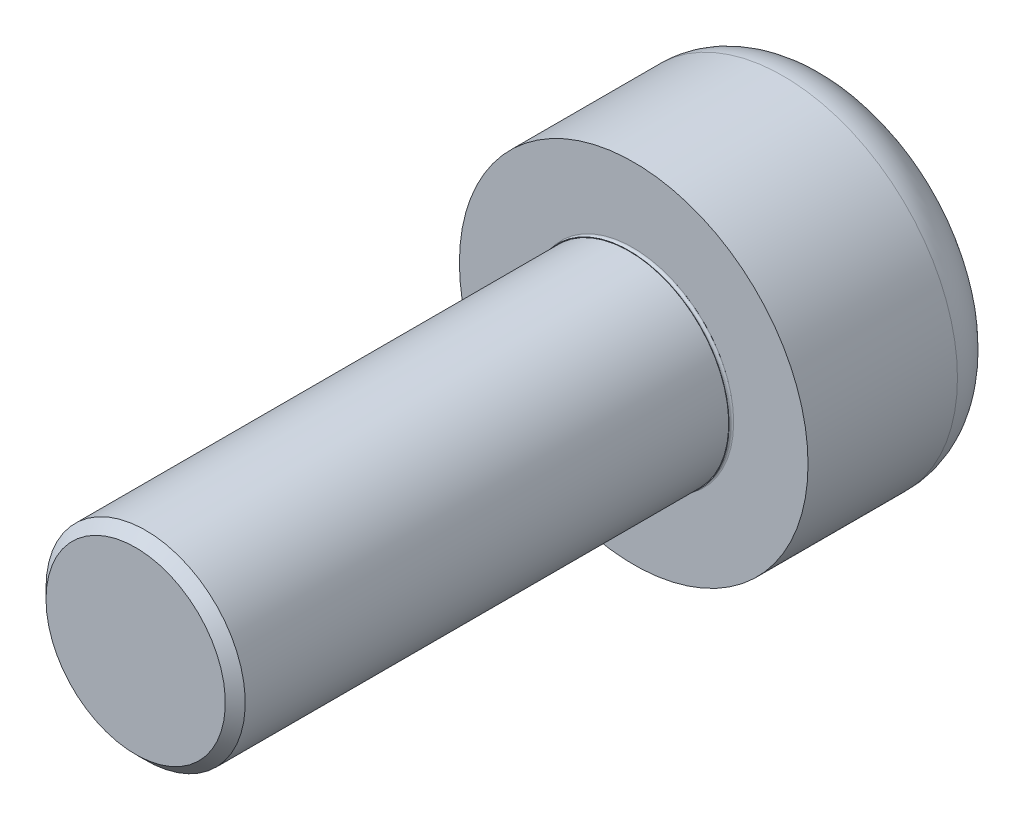
from build123d import *

# Parameters (mm, degrees)
CUT_EXTRUDE1_DEPTH = 0.75


with BuildPart() as part:
    # Logo3_bib1 → Revolve1 (revolve)
    with BuildSketch(Plane(origin=(0, 0, 0), x_dir=(-1, 0, 0), z_dir=(0, -1, 0))):
        with BuildLine():
            Line((0, -5), (0, 2))
            Line((0, 2), (1.25, 2))
            ThreePointArc((1.25, 2), (1.603553391, 1.853553391), (1.75, 1.5))
            Line((1.75, 1.5), (1.75, 0))
            Line((1.75, 0), (1, 0))
            Line((1, 0), (1, -0.01))
            Line((1, -0.01), (1.013425636, -0.01))
            ThreePointArc((1.013425636, -0.01), (0.993729481, -0.026527036), (1.006585234, -0.048793852))
            Line((1.006585234, -0.048793852), (1, -0.046397023))
            Line((1, -0.046397023), (1, -4.9))
            Line((1, -4.9), (0.9, -5))
            Line((0.9, -5), (0, -5))
        make_face()
    revolve(axis=Axis((0, 0, -10.585154653), (0, 0, 1)))

    # Logo3_bib2 → Cut-Extrude1 (cut)
    with BuildSketch(Plane(origin=(0, 0, -2), x_dir=(1, 0, 0), z_dir=(0, 0, -1))):
        Polygon((0.866025404, 0), (0.433012702, 0.75), (-0.433012702, 0.75), (-0.866025404, 0), (-0.433012702, -0.75), (0.433012702, -0.75), align=None)
    extrude(amount=-CUT_EXTRUDE1_DEPTH, mode=Mode.SUBTRACT)


solid = part.part
